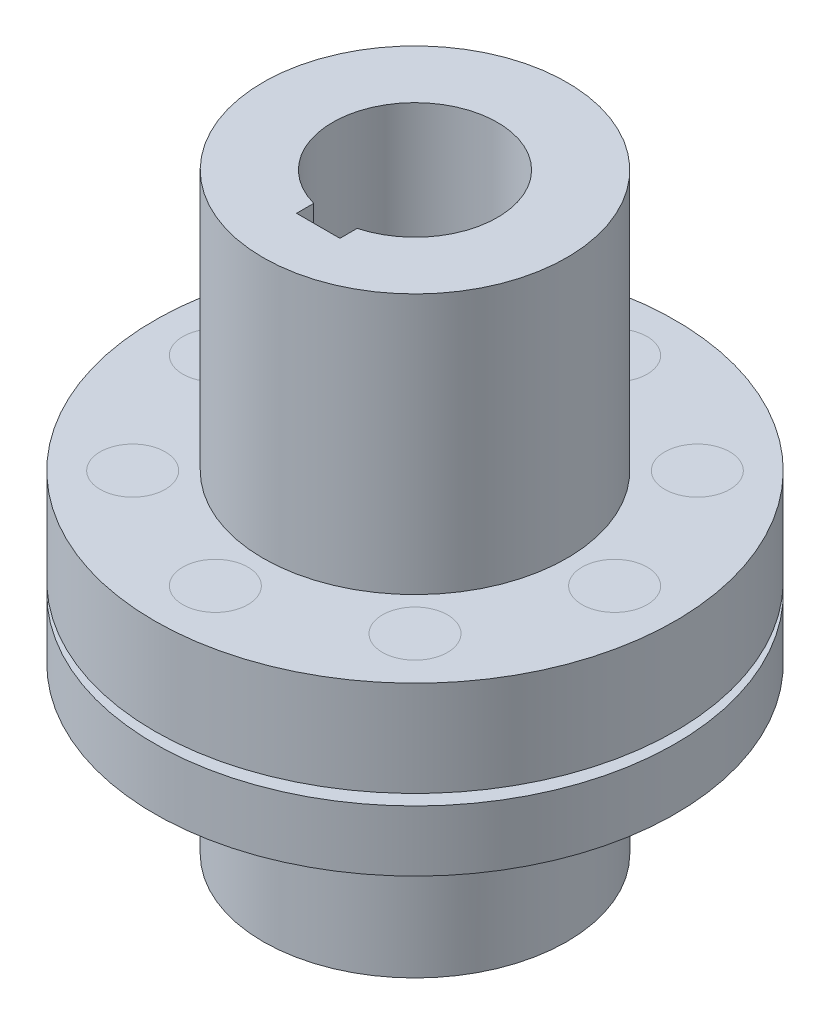
from build123d import *

# Parameters (mm, degrees)
SKETCH_2_R             = 7.5
CUT_EXTRUDE_1_DEPTH    = 104.923048454
SKETCH_3_R             = 7.5
BOSS_EXTRUDE_1_DEPTH   = 38.5
BOSS_EXTRUDE_1_2_DEPTH = 38.5
BOSS_EXTRUDE_1_3_DEPTH = 38.5
BOSS_EXTRUDE_1_4_DEPTH = 38.5
BOSS_EXTRUDE_1_5_DEPTH = 38.5
BOSS_EXTRUDE_1_6_DEPTH = 38.5
BOSS_EXTRUDE_1_7_DEPTH = 38.5
BOSS_EXTRUDE_1_8_DEPTH = 38.5
BOSS_EXTRUDE_START     = 2.5
SKETCH_4_R             = 60
SKETCH_4_R_2           = 7.5
SKETCH_4_R_3           = 10
BOSS_EXTRUDE_2_DEPTH   = 14
BOSS_EXTRUDE_START_2   = 38
SKETCH_5_R             = 35
SKETCH_5_R_2           = 10
BOSS_EXTRUDE_3_DEPTH   = 38
CUT_EXTRUDE_2_DEPTH    = 52
CUT_EXTRUDE_3_DEPTH    = 67


with BuildPart() as part:
    # Sketch 1 → Revolve 1 (revolve)
    with BuildSketch(Plane.XY, mode=Mode.PRIVATE) as revolve_1_sk:
        Polygon((-19, 15), (-19, 82), (-35, 82), (-35, 22), (-60, 22), (-60, 0), (-24, 0), (-24, 15), align=None)
    revolve(revolve_1_sk.sketch.rotate(Axis((0, 116.572916667, 0), (0, -1, 0)), 270), axis=Axis((0, 116.572916667, 0), (0, -1, 0)))

    # Sketch 2 → Cut-Extrude 1 (cut, through all)
    with BuildSketch(Plane(origin=(0, 22, 0), x_dir=(1, 0, 0), z_dir=(0, 1, 0))):
        with Locations(Location((0, -46, 0), (0, 0, 270))):
            Circle(SKETCH_2_R)
        with Locations(Location((-32.526911935, -32.526911935, 0), (0, 0, 270))):
            Circle(SKETCH_2_R)
        with Locations(Location((-46, 0, 0), (0, 0, 270))):
            Circle(SKETCH_2_R)
        with Locations(Location((-32.526911935, 32.526911935, 0), (0, 0, 270))):
            Circle(SKETCH_2_R)
        with Locations(Location((0, 46, 0), (0, 0, 270))):
            Circle(SKETCH_2_R)
        with Locations(Location((32.526911935, 32.526911935, 0), (0, 0, 270))):
            Circle(SKETCH_2_R)
        with Locations(Location((46, 0, 0), (0, 0, 270))):
            Circle(SKETCH_2_R)
        with Locations(Location((32.526911935, -32.526911935, 0), (0, 0, 270))):
            Circle(SKETCH_2_R)
    extrude(amount=-CUT_EXTRUDE_1_DEPTH, mode=Mode.SUBTRACT)

    # Sketch 7 → Cut-Extrude 3 (cut)
    with BuildSketch(Plane(origin=(0, 82, 0), x_dir=(1, 0, 0), z_dir=(0, 1, 0))):
        with BuildLine():
            Line((5, -18.33030278), (5, -22.3))
            Line((5, -22.3), (-5, -22.3))
            Line((-5, -22.3), (-5, -18.33030278))
            ThreePointArc((-5, -18.33030278), (0, -19), (5, -18.33030278))
        make_face()
    extrude(amount=-CUT_EXTRUDE_3_DEPTH, mode=Mode.SUBTRACT)


with BuildPart() as body_2:
    # Sketch 3 → Boss-Extrude 1 (new body)
    with BuildSketch(Plane(origin=(0, 22, 0), x_dir=(1, 0, 0), z_dir=(0, 1, 0))):
        with Locations(Location((0, -46, 0), (0, 0, 270))):
            Circle(SKETCH_3_R)
    extrude(amount=-BOSS_EXTRUDE_1_DEPTH)


with BuildPart() as body_3:
    # Sketch 3 → Boss-Extrude 1 2 (new body)
    with BuildSketch(Plane(origin=(0, 22, 0), x_dir=(1, 0, 0), z_dir=(0, 1, 0))):
        with Locations(Location((-32.526911935, -32.526911935, 0), (0, 0, 270))):
            Circle(SKETCH_3_R)
    extrude(amount=-BOSS_EXTRUDE_1_2_DEPTH)



with BuildPart() as body_4:
    # Sketch 3 → Boss-Extrude 1 3 (new body)
    with BuildSketch(Plane(origin=(0, 22, 0), x_dir=(1, 0, 0), z_dir=(0, 1, 0))):
        with Locations(Location((-46, 0, 0), (0, 0, 270))):
            Circle(SKETCH_3_R)
    extrude(amount=-BOSS_EXTRUDE_1_3_DEPTH)


with BuildPart() as body_5:
    # Sketch 3 → Boss-Extrude 1 4 (new body)
    with BuildSketch(Plane(origin=(0, 22, 0), x_dir=(1, 0, 0), z_dir=(0, 1, 0))):
        with Locations(Location((-32.526911935, 32.526911935, 0), (0, 0, 270))):
            Circle(SKETCH_3_R)
    extrude(amount=-BOSS_EXTRUDE_1_4_DEPTH)


with BuildPart() as body_6:
    # Sketch 3 → Boss-Extrude 1 5 (new body)
    with BuildSketch(Plane(origin=(0, 22, 0), x_dir=(1, 0, 0), z_dir=(0, 1, 0))):
        with Locations(Location((0, 46, 0), (0, 0, 270))):
            Circle(SKETCH_3_R)
    extrude(amount=-BOSS_EXTRUDE_1_5_DEPTH)


with BuildPart() as body_7:
    # Sketch 3 → Boss-Extrude 1 6 (new body)
    with BuildSketch(Plane(origin=(0, 22, 0), x_dir=(1, 0, 0), z_dir=(0, 1, 0))):
        with Locations(Location((32.526911935, 32.526911935, 0), (0, 0, 270))):
            Circle(SKETCH_3_R)
    extrude(amount=-BOSS_EXTRUDE_1_6_DEPTH)


with BuildPart() as body_8:
    # Sketch 3 → Boss-Extrude 1 7 (new body)
    with BuildSketch(Plane(origin=(0, 22, 0), x_dir=(1, 0, 0), z_dir=(0, 1, 0))):
        with Locations(Location((46, 0, 0), (0, 0, 270))):
            Circle(SKETCH_3_R)
    extrude(amount=-BOSS_EXTRUDE_1_7_DEPTH)


with BuildPart() as body_9:
    # Sketch 3 → Boss-Extrude 1 8 (new body)
    with BuildSketch(Plane(origin=(0, 22, 0), x_dir=(1, 0, 0), z_dir=(0, 1, 0))):
        with Locations(Location((32.526911935, -32.526911935, 0), (0, 0, 270))):
            Circle(SKETCH_3_R)
    extrude(amount=-BOSS_EXTRUDE_1_8_DEPTH)


with BuildPart() as body_10:
    # Sketch 4 → Boss-Extrude 2 (new body)
    with BuildSketch(Plane.XZ.offset(BOSS_EXTRUDE_START)):
        with Locations(Location((0, 0, 0), (0, 0, 90))):
            Circle(SKETCH_4_R)
        with Locations(Location((-32.526911935, 32.526911935, 0), (0, 0, 90))):
            Circle(SKETCH_4_R_2, mode=Mode.SUBTRACT)
        with Locations(Location((-46, 0, 0), (0, 0, 90))):
            Circle(SKETCH_4_R_2, mode=Mode.SUBTRACT)
        with Locations(Location((-32.526911935, -32.526911935, 0), (0, 0, 90))):
            Circle(SKETCH_4_R_2, mode=Mode.SUBTRACT)
        with Locations(Location((0, -46, 0), (0, 0, 90))):
            Circle(SKETCH_4_R_2, mode=Mode.SUBTRACT)
        with Locations(Location((32.526911935, -32.526911935, 0), (0, 0, 90))):
            Circle(SKETCH_4_R_2, mode=Mode.SUBTRACT)
        with Locations(Location((46, 0, 0), (0, 0, 90))):
            Circle(SKETCH_4_R_2, mode=Mode.SUBTRACT)
        with Locations(Location((32.526911935, 32.526911935, 0), (0, 0, 90))):
            Circle(SKETCH_4_R_2, mode=Mode.SUBTRACT)
        with Locations(Location((0, 46, 0), (0, 0, 90))):
            Circle(SKETCH_4_R_2, mode=Mode.SUBTRACT)
        with Locations(Location((0, 0, 0), (0, 0, 270))):
            Circle(SKETCH_4_R_3, mode=Mode.SUBTRACT)
    extrude(amount=BOSS_EXTRUDE_2_DEPTH)


with BuildPart() as body_3_1:
    add(body_3.part)

    add(body_10.part)  # Boss-Extrude 3 merges body 10

    add(body_5.part)  # Boss-Extrude 3 merges body 5

    add(body_7.part)  # Boss-Extrude 3 merges body 7

    add(body_9.part)  # Boss-Extrude 3 merges body 9
    # Sketch 5 → Boss-Extrude 3 (add)
    with BuildSketch(Plane.XZ.offset(16.5).offset(BOSS_EXTRUDE_START_2)):
        with Locations(Location((0, 0, 0), (0, 0, 90))):
            Circle(SKETCH_5_R)
        with Locations(Location((0, 0, 0), (0, 0, 270))):
            Circle(SKETCH_5_R_2, mode=Mode.SUBTRACT)
    extrude(amount=-BOSS_EXTRUDE_3_DEPTH)

    # Sketch 6 → Cut-Extrude 2 (cut)
    with BuildSketch(Plane.XZ.offset(54.5)):
        with BuildLine():
            Line((-3, 9.539392014), (-3, 12.8))
            Line((-3, 12.8), (3, 12.8))
            Line((3, 12.8), (3, 9.539392014))
            ThreePointArc((3, 9.539392014), (0, 10), (-3, 9.539392014))
        make_face()
    extrude(amount=-CUT_EXTRUDE_2_DEPTH, mode=Mode.SUBTRACT)


solid = Compound([part.part, body_2.part, body_4.part, body_6.part, body_8.part, body_3_1.part])
